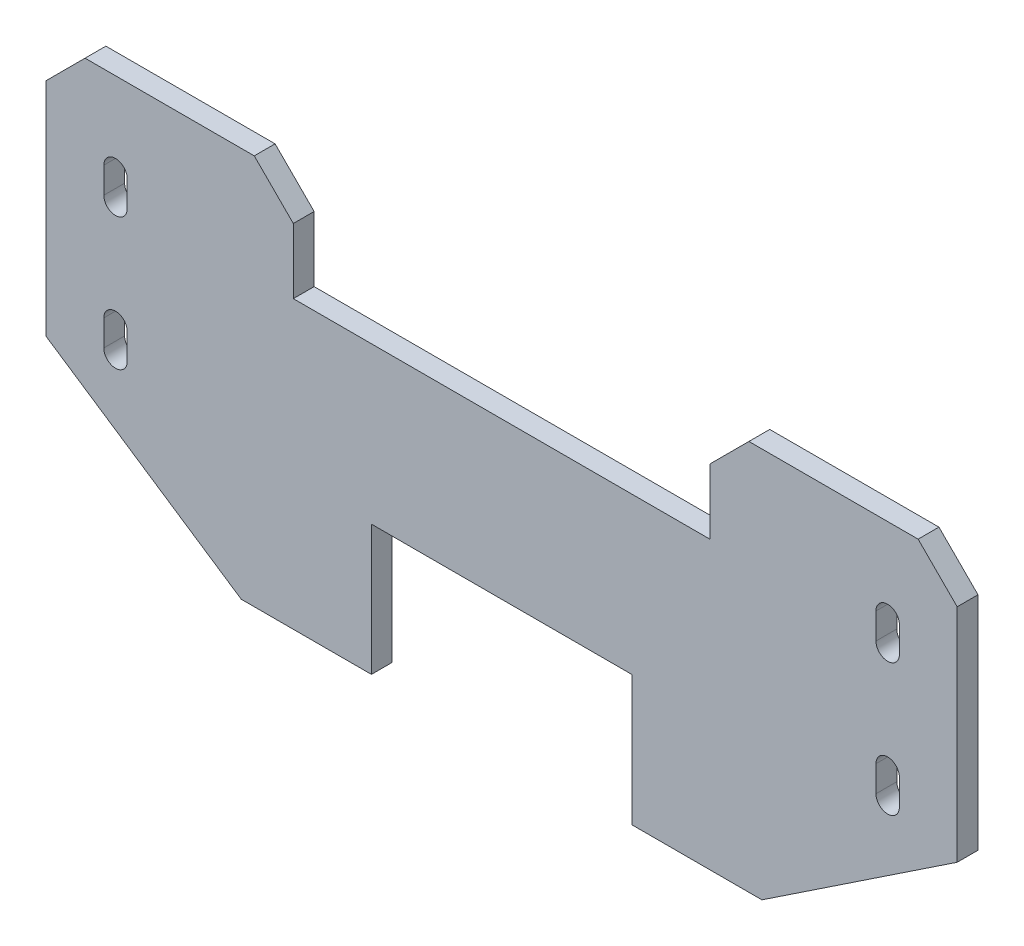
from build123d import *

# Parameters (mm, degrees)
EXTRUDE_1_DEPTH = 8


with BuildPart() as part:
    # 草图1 → 凸台-拉伸1 (new body)
    with BuildSketch(Plane.XY):
        Polygon((175, -25), (100, -75), (50, -75), (50, -25), (-50, -25), (-50, -75), (-100, -75), (-175, -25), (-175, 60), (-160, 75), (-95, 75), (-80, 60), (-80, 35), (80, 35), (80, 60), (95, 75), (160, 75), (175, 60), align=None)
        with BuildLine():
            Line((-143.8, 43), (-143.8, 33))
            ThreePointArc((-143.8, 33), (-148.3, 28.5), (-152.8, 33))
            Line((-152.8, 33), (-152.8, 43))
            ThreePointArc((-152.8, 43), (-148.3, 47.5), (-143.8, 43))
        make_face(mode=Mode.SUBTRACT)
        with BuildLine():
            Line((-143.8, -7.8), (-143.8, -17.8))
            ThreePointArc((-143.8, -17.8), (-148.3, -22.3), (-152.8, -17.8))
            Line((-152.8, -17.8), (-152.8, -7.8))
            ThreePointArc((-152.8, -7.8), (-148.3, -3.3), (-143.8, -7.8))
        make_face(mode=Mode.SUBTRACT)
        with BuildLine():
            Line((143.8, -7.8), (143.8, -17.8))
            ThreePointArc((143.8, -17.8), (148.3, -22.3), (152.8, -17.8))
            Line((152.8, -17.8), (152.8, -7.8))
            ThreePointArc((152.8, -7.8), (148.3, -3.3), (143.8, -7.8))
        make_face(mode=Mode.SUBTRACT)
        with BuildLine():
            Line((143.8, 43), (143.8, 33))
            ThreePointArc((143.8, 33), (148.3, 28.5), (152.8, 33))
            Line((152.8, 33), (152.8, 43))
            ThreePointArc((152.8, 43), (148.3, 47.5), (143.8, 43))
        make_face(mode=Mode.SUBTRACT)
    extrude(amount=EXTRUDE_1_DEPTH)


solid = part.part
